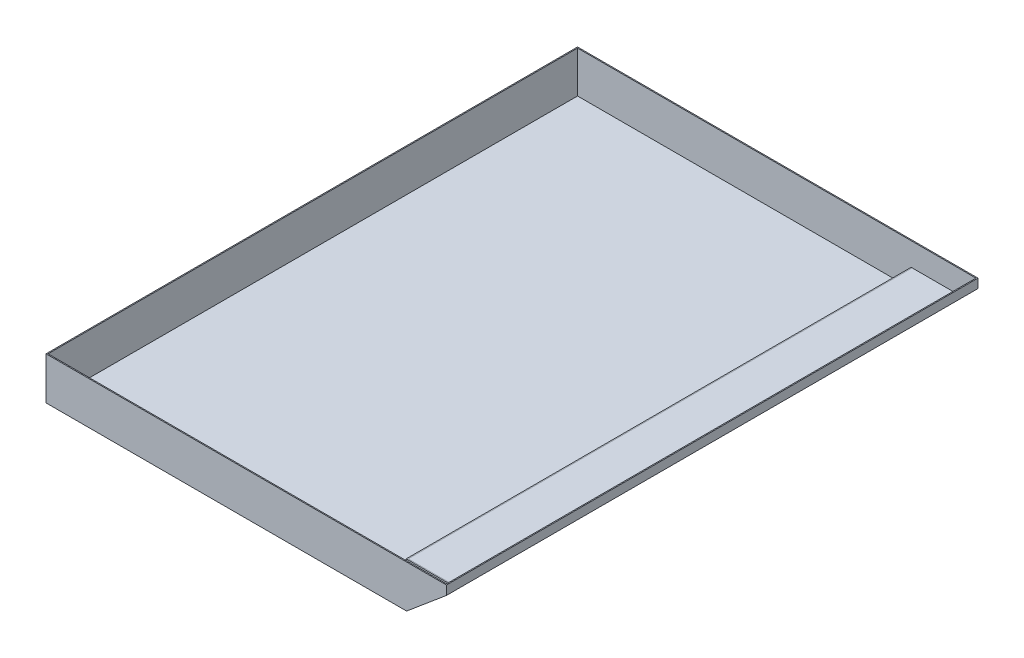
SolidWorks part; units mm, degrees
ref_plane "前视基准面" through (0, 0, 0) normal (0, 0, 1) x (1, 0, 0)
ref_plane "上视基准面" through (0, 0, 0) normal (0, 1, 0) x (1, 0, 0)
ref_plane "右视基准面" through (0, 0, 0) normal (1, 0, 0) x (0, 0, -1)
sketch "草图2" plane through (0, 0, 0) normal (0, 0, 1) x (1, 0, 0)
  line L0 (0, 0) -> (0, 83)
  line L1 (0, 83) -> (784, 83)
  line L3 (784, 67) -> (704.1525, 0)
  line L4 (704.1525, 0) -> (0, 0)
  line L5 (784, 83) -> (784, 67)
  dimension "D1" = 67
  dimension "D2" = 140
  dimension "D3" = 784
  dimension "D4" = 83
extrude "凸台-拉伸1" add sketch "草图2" along normal blind 1038
sketch "草图8" plane through (0, 0, 1038) normal (0, 0, 1) x (1, 0, 0)
  line L0 (784, 67) -> (784, 83) construction
  line L1 (782, 134.1526) -> (892.0044, 134.1526)
  line L2 (782, 134.1526) -> (782, 0)
  line L3 (782, 0) -> (892.0044, 0)
  line L4 (892.0044, 134.1526) -> (892.0044, 0)
  dimension "D1" = 2
extrude "切除-拉伸2" cut sketch "草图8" against normal blind 1191
shell "抽壳1" thickness 2
sketch "草图3" plane through (290.9389, -346.7274, 0) normal (0.6428, -0.766, 0) x (0.766, 0.6428, 0)
  line L0 (539.4121, 519) -> (815.6504, 519) construction
  line L1 (539.4121, 1038) -> (539.4121, 0) construction
  line L2 (590.2235, 1038) -> (590.2235, -41.4419) construction
  line L3 (539.4121, 1038) -> (641.0348, 1038) construction
  line L5 (552.7235, 1010) -> (627.7235, 1010)
  line L6 (552.7235, 1010) -> (552.7235, 28)
  line L7 (552.7235, 28) -> (627.7235, 28)
  line L8 (627.7235, 1010) -> (627.7235, 28)
  dimension "D1" = 491
  dimension "D2" = 982
  dimension "D3" = 37.5
  dimension "D4" = 75
extrude "切除-拉伸1" cut sketch "草图3" against normal blind 654
sketch "草图5" plane through (0, 2, 0) normal (0, 1, 0) x (1, 0, 0)
  line L0 (2, -519) -> (979.0478, -519) construction
  line L1 (677.4246, -26) -> (679.4246, -26)
  line L2 (677.4246, -26) -> (677.4246, -1012)
  line L3 (677.4246, -1012) -> (679.4246, -1012)
  line L4 (679.4246, -26) -> (679.4246, -1012)
  line L5 (2, -1036) -> (2, -2) construction
  line L6 (703.4246, -1036) -> (703.4246, -2) construction
  dimension "D1" = 2
  dimension "D2" = 24
  dimension "D3" = 986
  dimension "D4" = 493
extrude "凸台-拉伸2" add sketch "草图5" along normal blind 60
ref_plane "基准面1" through (0, 0, 519) normal (0, 0, 1) x (1, 0, 0)
sketch "草图6" plane through (0, 0, 519) normal (0, 0, 1) x (1, 0, 0)
  line L0 (679.4246, 62) -> (774.9298, 62)
  line L1 (703.4246, 2) -> (780, 66.2544) construction
  line L2 (774.9298, 62) -> (772.5463, 60)
  line L16 (681.4246, 62) -> (681.4246, 2)
  line L17 (681.4246, 60) -> (681.4246, 4)
  line L21 (681.4246, 60) -> (772.5463, 60)
  line L22 (702.139, 3.5321) -> (778.7144, 67.7865)
  line L23 (702.6966, 4) -> (746.2504, 40.546)
  line L24 (679.4246, 62) -> (679.4246, 2)
  line L25 (679.4246, 2) -> (703.4246, 2)
  line L26 (703.4246, 2) -> (747.536, 39.0139)
  line L27 (747.536, 39.0139) -> (746.2504, 40.546)
  line L28 (681.4246, 4) -> (702.6966, 4)
  line L29 (679.4246, 60) -> (774.9298, 60) construction
  line L30 (770.5173, 58.2975) -> (771.8029, 56.7654) construction
  dimension "D2" = 2
  dimension "D5" = 30
  dimension "D1" = 2
  dimension "D3" = 2
  dimension "D4" = 2
extrude "凸台-拉伸3" add sketch "草图6" along normal blind 493 and the other way blind 493 separate body
sketch "草图9" plane through (0, 0, 1012) normal (0, 0, 1) x (1, 0, 0)
  line L0 (679.4246, 62) -> (679.4246, 2)
  line L1 (679.4246, 2) -> (703.4246, 2)
  line L2 (703.4246, 2) -> (774.9298, 62)
  line L3 (774.9298, 62) -> (679.4246, 62)
extrude "凸台-拉伸5" add sketch "草图9" against normal blind 2 separate body
sketch "草图10" plane through (0, 0, 26) normal (0, 0, -1) x (-1, 0, 0)
  line L0 (-679.4246, 2) -> (-679.4246, 62)
  line L1 (-679.4246, 62) -> (-774.9298, 62)
  line L2 (-774.9298, 62) -> (-703.4246, 2)
  line L3 (-703.4246, 2) -> (-679.4246, 2)
extrude "凸台-拉伸6" add sketch "草图10" against normal blind 2 separate body
